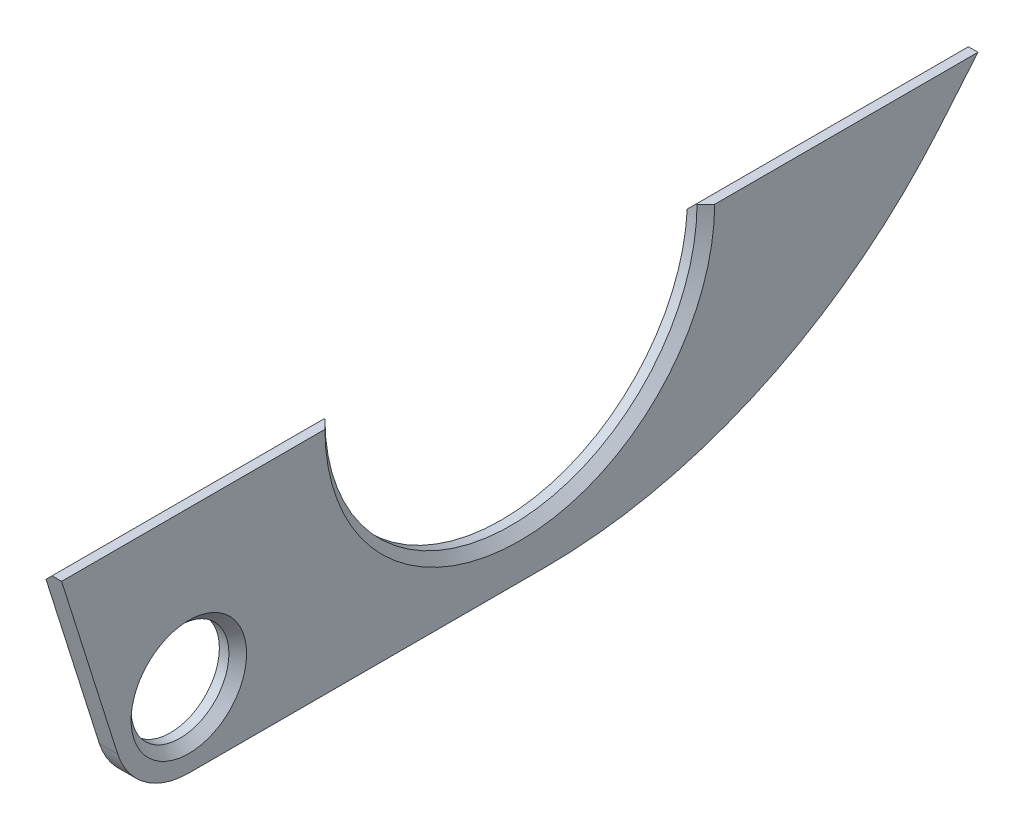
SolidWorks part; units mm, degrees
material "Q345B"
ref_plane "Front Plane" through (0, 0, 0) normal (0, 0, 1) x (1, 0, 0)
ref_plane "Top Plane" through (0, 0, 0) normal (0, 1, 0) x (1, 0, 0)
ref_plane "Right Plane" through (0, 0, 0) normal (1, 0, 0) x (0, 0, -1)
sketch "Sketch1" plane through (0, 0, 0) normal (1, 0, 0) x (0, 0, -1)
  line L0 (-55.2907, 0) -> (73.0254, 0) construction
  line L1 (0, 67.5426) -> (0, -31.3548) construction
  line L2 (623, -1.2) -> (252.9972, -1.2)
  line L3 (-623, -1.2) -> (-546.7897, -242.5615)
  line L6 (-450, -313.5) -> (360.9492, -313.5)
  line L7 (360.9492, -313.5) -> (623, -1.2)
  line L11 (-252.9972, -1.2) -> (-623, -1.2)
  arc A0 (-252.9972, -1.2) -> (252.9972, -1.2) centre (0, 0) ccw
  arc A2 (-546.7897, -242.5615) -> (-450, -313.5) centre (-450, -212) ccw
  dimension "D1" = 506
  dimension "D2" = 101.5
  dimension "D3" = 50
  dimension "D4" = 623
  dimension "D5" = 1.2
  dimension "D6" = 623
  dimension "D14" = 450
  dimension "D15" = 212
extrude "Boss-Extrude1" add sketch "Sketch1" along normal mid plane 25
sketch "Sketch2" plane through (0, 0, 0) normal (1, 0, 0) x (0, 0, -1)
  circle A1 centre (-450, -212) radius 66.5
  dimension "D1" = 133
extrude "Cut-Extrude1" cut sketch "Sketch2" against normal through all both and the other way through all
fillet "Fillet1" radius 700 1 edges at (0, -313.5, -360.9492)
chamfer "Chamfer1" distance 12 angle 45 2 edges at (12.5, -253, 0) (12.5, -212, 383.5)
chamfer "Chamfer2" distance 12 angle 45 2 edges at (-12.5, -1.2, -437.9986) (-12.5, -1.2, 437.9986)
